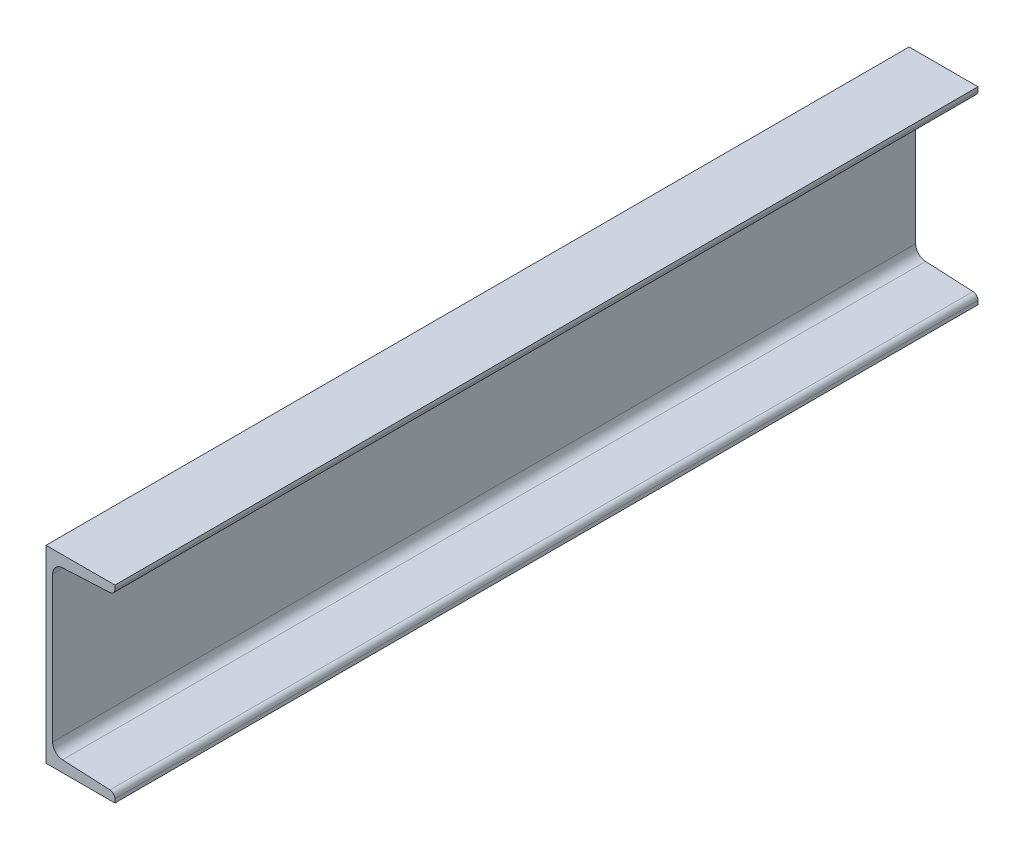
from build123d import *

# Parameters (mm, degrees)
BOSS_EXTRUDE1_DEPTH = 457.2


with BuildPart() as part:
    # Sketch1 → Boss-Extrude1 (new, symmetric)
    with BuildSketch(Plane(origin=(28.211262136, 0, 0), x_dir=(-1, 0, 0), z_dir=(0, 0, 1))):
        with BuildLine():
            Line((28.211262136, 0), (28.211262136, -200))
            Line((28.211262136, -200), (-44.788737864, -200))
            Line((-44.788737864, -200), (-44.788737864, -196.033179359))
            ThreePointArc((-44.788737864, -196.033179359), (-43.272315441, -192.240936001), (-39.559243433, -190.539835501))
            Line((-39.559243433, -190.539835501), (10.752273273, -188.062374452))
            ThreePointArc((10.752273273, -188.062374452), (18.17841729, -184.660173452), (21.211262136, -177.075686736))
            Line((21.211262136, -177.075686736), (21.211262136, -22.924313264))
            ThreePointArc((21.211262136, -22.924313264), (18.17841729, -15.339826548), (10.752273273, -11.937625548))
            Line((10.752273273, -11.937625548), (-39.559243433, -9.460164499))
            ThreePointArc((-39.559243433, -9.460164499), (-43.272315441, -7.759063999), (-44.788737864, -3.966820641))
            Line((-44.788737864, -3.966820641), (-44.788737864, 0))
            Line((-44.788737864, 0), (28.211262136, 0))
        make_face()
    extrude(amount=BOSS_EXTRUDE1_DEPTH, both=True)


solid = part.part
